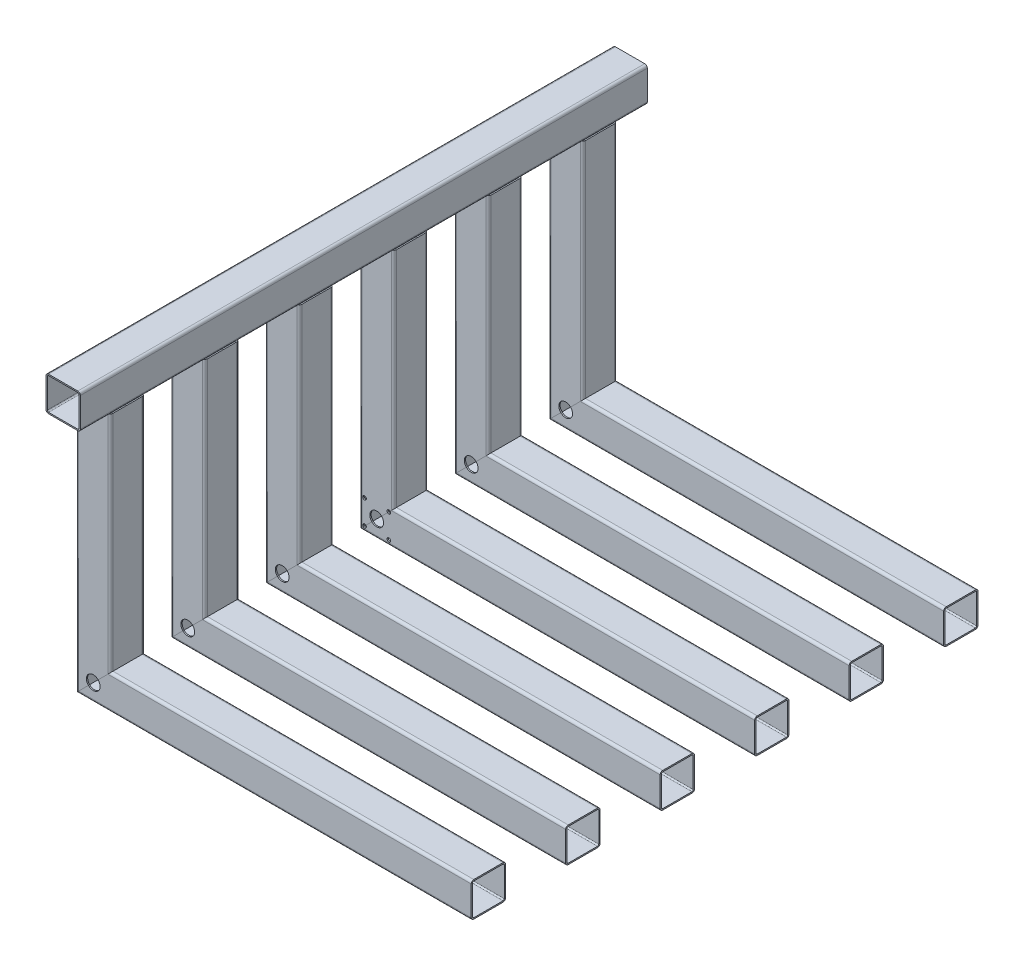
from build123d import *

# Parameters (mm, degrees)
GB_T6728_2002_40_X_40_X_1_5_1_DEPTH   = 660
GB_T6728_2002_40_X_40_X_1_5_1_2_DEPTH = 330.284271247
GB_T6728_2002_40_X_40_X_1_5_1_3_DEPTH = 469.284271247
PATTERN_LINEAR_1_COUNT                = 6
PATTERN_LINEAR_1_PITCH                = 110
SKETCH_2_R                            = 8
CUT_EXTRUDE_1_DEPTH                   = 743.041103983
SKETCH_5_W                            = 2.1
SKETCH_5_H                            = 1.501
PATTERN_CIRCULAR_1_COUNT              = 4
MIRROR_2_COPY_1_SKETCH_W              = 2.1
MIRROR_2_COPY_1_SKETCH_H              = 1.501
MIRROR_2_COPY_2_SKETCH_W              = 2.1
MIRROR_2_COPY_2_SKETCH_H              = 1.501
MIRROR_2_COPY_3_SKETCH_W              = 2.1
MIRROR_2_COPY_3_SKETCH_H              = 1.501


with BuildPart() as part:
    # Sketch1 → 冷弯空心方管gb∕t6728-2002 40 X 40 X 1.5(1) (new body)
    with BuildSketch(Plane(origin=(-220, 300, 330), x_dir=(1, 0, 0), z_dir=(0, 0, -1))):
        with BuildLine():
            Line((-17, -20), (17, -20))
            ThreePointArc((17, -20), (19.121320344, -19.121320344), (20, -17))
            Line((20, -17), (20, 17))
            ThreePointArc((20, 17), (19.121320344, 19.121320344), (17, 20))
            Line((17, 20), (-17, 20))
            ThreePointArc((-17, 20), (-19.121320344, 19.121320344), (-20, 17))
            Line((-20, 17), (-20, -17))
            ThreePointArc((-20, -17), (-19.121320344, -19.121320344), (-17, -20))
        make_face()
        with BuildLine():
            Line((-17, -18.5), (17, -18.5))
            ThreePointArc((17, -18.5), (18.060660172, -18.060660172), (18.5, -17))
            Line((18.5, -17), (18.5, 17))
            ThreePointArc((18.5, 17), (18.060660172, 18.060660172), (17, 18.5))
            Line((17, 18.5), (-17, 18.5))
            ThreePointArc((-17, 18.5), (-18.060660172, 18.060660172), (-18.5, 17))
            Line((-18.5, 17), (-18.5, -17))
            ThreePointArc((-18.5, -17), (-18.060660172, -18.060660172), (-17, -18.5))
        make_face(mode=Mode.SUBTRACT)
    extrude(amount=GB_T6728_2002_40_X_40_X_1_5_1_DEPTH)


with BuildPart() as body_2:
    # Sketch1 on segment 2 (carried to segment 2) → gb_t6728-2002 40 X 40 X 1.5_1 2 (new body)
    with BuildSketch(Plane(origin=(-220, 301, 275), x_dir=(1, 0, 0), z_dir=(0, -1, 0))):
        with BuildLine():
            Line((-17, -20), (17, -20))
            ThreePointArc((17, -20), (19.121320344, -19.121320344), (20, -17))
            Line((20, -17), (20, 17))
            ThreePointArc((20, 17), (19.121320344, 19.121320344), (17, 20))
            Line((17, 20), (-17, 20))
            ThreePointArc((-17, 20), (-19.121320344, 19.121320344), (-20, 17))
            Line((-20, 17), (-20, -17))
            ThreePointArc((-20, -17), (-19.121320344, -19.121320344), (-17, -20))
        make_face()
        with BuildLine():
            Line((-17, -18.5), (17, -18.5))
            ThreePointArc((17, -18.5), (18.060660172, -18.060660172), (18.5, -17))
            Line((18.5, -17), (18.5, 17))
            ThreePointArc((18.5, 17), (18.060660172, 18.060660172), (17, 18.5))
            Line((17, 18.5), (-17, 18.5))
            ThreePointArc((-17, 18.5), (-18.060660172, 18.060660172), (-18.5, 17))
            Line((-18.5, 17), (-18.5, -17))
            ThreePointArc((-18.5, -17), (-18.060660172, -18.060660172), (-17, -18.5))
        make_face(mode=Mode.SUBTRACT)
    extrude(amount=GB_T6728_2002_40_X_40_X_1_5_1_2_DEPTH)

    # gb_t6728-2002 40 X 40 X 1.5_1 2 mitre 1
    split(bisect_by=Plane(origin=(-220, 0, 275), x_dir=(-0.707106781, -0.707106781, 0), z_dir=(-0.707106781, 0.707106781, 0)), keep=Keep.TOP)

    # gb_t6728-2002 40 X 40 X 1.5_1 2 mitre 2
    split(bisect_by=Plane(origin=(-220, 280, 275), x_dir=(1, 0, 0), z_dir=(0, -1, 0)), keep=Keep.TOP)


with BuildPart() as body_3:
    # Sketch1 on segment 3 (carried to segment 3) → gb_t6728-2002 40 X 40 X 1.5_1 3 (new body)
    with BuildSketch(Plane(origin=(-249.284271247, 0, 275), x_dir=(0, 0, 1), z_dir=(1, 0, 0))):
        with BuildLine():
            Line((-17, -20), (17, -20))
            ThreePointArc((17, -20), (19.121320344, -19.121320344), (20, -17))
            Line((20, -17), (20, 17))
            ThreePointArc((20, 17), (19.121320344, 19.121320344), (17, 20))
            Line((17, 20), (-17, 20))
            ThreePointArc((-17, 20), (-19.121320344, 19.121320344), (-20, 17))
            Line((-20, 17), (-20, -17))
            ThreePointArc((-20, -17), (-19.121320344, -19.121320344), (-17, -20))
        make_face()
        with BuildLine():
            Line((-17, -18.5), (17, -18.5))
            ThreePointArc((17, -18.5), (18.060660172, -18.060660172), (18.5, -17))
            Line((18.5, -17), (18.5, 17))
            ThreePointArc((18.5, 17), (18.060660172, 18.060660172), (17, 18.5))
            Line((17, 18.5), (-17, 18.5))
            ThreePointArc((-17, 18.5), (-18.060660172, 18.060660172), (-18.5, 17))
            Line((-18.5, 17), (-18.5, -17))
            ThreePointArc((-18.5, -17), (-18.060660172, -18.060660172), (-17, -18.5))
        make_face(mode=Mode.SUBTRACT)
    extrude(amount=GB_T6728_2002_40_X_40_X_1_5_1_3_DEPTH)

    # gb_t6728-2002 40 X 40 X 1.5_1 3 mitre 1
    split(bisect_by=Plane(origin=(-220, 0, 275), x_dir=(0.707106781, 0.707106781, 0), z_dir=(0.707106781, -0.707106781, 0)), keep=Keep.TOP)


with BuildPart() as pattern_linear_1_1:
    # 阵列(线性)1: pattern copy
    add(body_3.part.moved(Location(Vector(0, 0, -1) * (1 * PATTERN_LINEAR_1_PITCH))))


with BuildPart() as pattern_linear_1_2:
    # 阵列(线性)1: pattern copy
    add(body_3.part.moved(Location(Vector(0, 0, -1) * (2 * PATTERN_LINEAR_1_PITCH))))


with BuildPart() as pattern_linear_1_3:
    # 阵列(线性)1: pattern copy
    add(body_3.part.moved(Location(Vector(0, 0, -1) * (3 * PATTERN_LINEAR_1_PITCH))))


with BuildPart() as pattern_linear_1_4:
    # 阵列(线性)1: pattern copy
    add(body_3.part.moved(Location(Vector(0, 0, -1) * (4 * PATTERN_LINEAR_1_PITCH))))


with BuildPart() as pattern_linear_1_5:
    # 阵列(线性)1: pattern copy
    add(body_3.part.moved(Location(Vector(0, 0, -1) * (5 * PATTERN_LINEAR_1_PITCH))))


with BuildPart() as pattern_linear_1_6:
    # 阵列(线性)1: pattern copy
    add(body_2.part.moved(Location(Vector(0, 0, -1) * (1 * PATTERN_LINEAR_1_PITCH))))


with BuildPart() as pattern_linear_1_7:
    # 阵列(线性)1: pattern copy
    add(body_2.part.moved(Location(Vector(0, 0, -1) * (2 * PATTERN_LINEAR_1_PITCH))))


with BuildPart() as pattern_linear_1_8:
    # 阵列(线性)1: pattern copy
    add(body_2.part.moved(Location(Vector(0, 0, -1) * (3 * PATTERN_LINEAR_1_PITCH))))


with BuildPart() as pattern_linear_1_9:
    # 阵列(线性)1: pattern copy
    add(body_2.part.moved(Location(Vector(0, 0, -1) * (4 * PATTERN_LINEAR_1_PITCH))))


with BuildPart() as pattern_linear_1_10:
    # 阵列(线性)1: pattern copy
    add(body_2.part.moved(Location(Vector(0, 0, -1) * (5 * PATTERN_LINEAR_1_PITCH))))


with BuildPart() as cut_extrude_1_tool:
    # Sketch 2 → 切除-拉伸1 (new, through all)
    with BuildSketch(Plane.XY.offset(295)):
        with Locations((-220, 0)):
            Circle(SKETCH_2_R)
    extrude(amount=-CUT_EXTRUDE_1_DEPTH)


with BuildPart() as body_2_1:
    add(body_2.part)

    # 切除-拉伸1: cut by cut_extrude_1_tool
    add(cut_extrude_1_tool.part, mode=Mode.SUBTRACT)


with BuildPart() as body_3_1:
    add(body_3.part)

    # 切除-拉伸1: cut by cut_extrude_1_tool
    add(cut_extrude_1_tool.part, mode=Mode.SUBTRACT)


with BuildPart() as pattern_linear_1_1_1:
    add(pattern_linear_1_1.part)

    # 切除-拉伸1: cut by cut_extrude_1_tool
    add(cut_extrude_1_tool.part, mode=Mode.SUBTRACT)


with BuildPart() as pattern_linear_1_2_1:
    add(pattern_linear_1_2.part)

    # 切除-拉伸1: cut by cut_extrude_1_tool
    add(cut_extrude_1_tool.part, mode=Mode.SUBTRACT)


with BuildPart() as pattern_linear_1_3_1:
    add(pattern_linear_1_3.part)

    # 切除-拉伸1: cut by cut_extrude_1_tool
    add(cut_extrude_1_tool.part, mode=Mode.SUBTRACT)


with BuildPart() as pattern_linear_1_4_1:
    add(pattern_linear_1_4.part)

    # 切除-拉伸1: cut by cut_extrude_1_tool
    add(cut_extrude_1_tool.part, mode=Mode.SUBTRACT)


with BuildPart() as pattern_linear_1_5_1:
    add(pattern_linear_1_5.part)

    # 切除-拉伸1: cut by cut_extrude_1_tool
    add(cut_extrude_1_tool.part, mode=Mode.SUBTRACT)


with BuildPart() as pattern_linear_1_6_1:
    add(pattern_linear_1_6.part)

    # 切除-拉伸1: cut by cut_extrude_1_tool
    add(cut_extrude_1_tool.part, mode=Mode.SUBTRACT)


with BuildPart() as pattern_linear_1_7_1:
    add(pattern_linear_1_7.part)

    # 切除-拉伸1: cut by cut_extrude_1_tool
    add(cut_extrude_1_tool.part, mode=Mode.SUBTRACT)


with BuildPart() as pattern_linear_1_8_1:
    add(pattern_linear_1_8.part)

    # 切除-拉伸1: cut by cut_extrude_1_tool
    add(cut_extrude_1_tool.part, mode=Mode.SUBTRACT)

    # 草图5 → M5 螺纹孔1 (revolve, cut)
    with BuildSketch(Plane(origin=(-234.142135624, 14.142135624, -35), x_dir=(0, -1, 0), z_dir=(1, 0, 0))):
        with Locations((1.05, 0.7505)):
            Rectangle(SKETCH_5_W, SKETCH_5_H)
    hole_wizard_m5_1 = revolve(axis=Axis((-234.142135624, 14.142135624, -28.65), (0, 0, -1)), mode=Mode.SUBTRACT)


with BuildPart() as pattern_linear_1_9_1:
    add(pattern_linear_1_9.part)

    # 切除-拉伸1: cut by cut_extrude_1_tool
    add(cut_extrude_1_tool.part, mode=Mode.SUBTRACT)


with BuildPart() as pattern_linear_1_10_1:
    add(pattern_linear_1_10.part)

    # 切除-拉伸1: cut by cut_extrude_1_tool
    add(cut_extrude_1_tool.part, mode=Mode.SUBTRACT)


with BuildPart() as pattern_circular_1_tool:
    # 阵列(圆周)1: M5 螺纹孔1 ×4 about axis
    pattern_circular_1_axis = Axis((-220, 0, 0), (0, 0, 1))
    for i in range(1, PATTERN_CIRCULAR_1_COUNT):
        add(hole_wizard_m5_1.rotate(pattern_circular_1_axis, i * 360 / PATTERN_CIRCULAR_1_COUNT))


with BuildPart() as pattern_linear_1_3_2:
    add(pattern_linear_1_3_1.part)

    # 阵列(圆周)1: cut by pattern_circular_1_tool
    add(pattern_circular_1_tool.part, mode=Mode.SUBTRACT)


with BuildPart() as pattern_linear_1_8_2:
    add(pattern_linear_1_8_1.part)

    # 阵列(圆周)1: cut by pattern_circular_1_tool
    add(pattern_circular_1_tool.part, mode=Mode.SUBTRACT)


with BuildPart() as pattern_linear_1_7_2:
    add(pattern_linear_1_7_1.part)

    # 镜向2: M5 螺纹孔1 across plane
    add(hole_wizard_m5_1.mirror(Plane.XY), mode=Mode.SUBTRACT)


with BuildPart() as mirror_2_copy_1_tool:
    # 镜向2 copy 1 sketch → 镜向2 copy 1 (revolve)
    with BuildSketch(Plane(origin=(-234.142135624, -14.142135624, 35), x_dir=(1, 0, 0), z_dir=(0, 1, 0))):
        with Locations((1.05, -0.7505)):
            Rectangle(MIRROR_2_COPY_1_SKETCH_W, MIRROR_2_COPY_1_SKETCH_H)
    revolve(axis=Axis((-234.142135624, -14.142135624, 28.65), (0, 0, -1)))


with BuildPart() as pattern_linear_1_2_2:
    add(pattern_linear_1_2_1.part)

    # 镜向2 copy 1: cut by mirror_2_copy_1_tool
    add(mirror_2_copy_1_tool.part, mode=Mode.SUBTRACT)

    # 镜向2 copy 2 sketch → 镜向2 copy 2 (revolve, cut)
    with BuildSketch(Plane(origin=(-205.857864376, -14.142135624, 35), x_dir=(0, 1, 0), z_dir=(-1, 0, 0))):
        with Locations((1.05, -0.7505)):
            Rectangle(MIRROR_2_COPY_2_SKETCH_W, MIRROR_2_COPY_2_SKETCH_H)
    revolve(axis=Axis((-205.857864376, -14.142135624, 28.65), (0, 0, -1)), mode=Mode.SUBTRACT)


with BuildPart() as pattern_linear_1_7_3:
    add(pattern_linear_1_7_2.part)

    # 镜向2 copy 1: cut by mirror_2_copy_1_tool
    add(mirror_2_copy_1_tool.part, mode=Mode.SUBTRACT)


with BuildPart() as mirror_2_copy_3_tool:
    # 镜向2 copy 3 sketch → 镜向2 copy 3 (revolve)
    with BuildSketch(Plane(origin=(-205.857864376, 14.142135624, 35), x_dir=(-1, 0, 0), z_dir=(0, -1, 0))):
        with Locations((1.05, -0.7505)):
            Rectangle(MIRROR_2_COPY_3_SKETCH_W, MIRROR_2_COPY_3_SKETCH_H)
    revolve(axis=Axis((-205.857864376, 14.142135624, 28.65), (0, 0, -1)))


with BuildPart() as pattern_linear_1_2_3:
    add(pattern_linear_1_2_2.part)

    # 镜向2 copy 3: cut by mirror_2_copy_3_tool
    add(mirror_2_copy_3_tool.part, mode=Mode.SUBTRACT)


with BuildPart() as pattern_linear_1_7_4:
    add(pattern_linear_1_7_3.part)

    # 镜向2 copy 3: cut by mirror_2_copy_3_tool
    add(mirror_2_copy_3_tool.part, mode=Mode.SUBTRACT)


solid = Compound([part.part, body_2_1.part, body_3_1.part, pattern_linear_1_1_1.part, pattern_linear_1_4_1.part, pattern_linear_1_5_1.part, pattern_linear_1_6_1.part, pattern_linear_1_9_1.part, pattern_linear_1_10_1.part, pattern_linear_1_3_2.part, pattern_linear_1_8_2.part, pattern_linear_1_2_3.part, pattern_linear_1_7_4.part])
